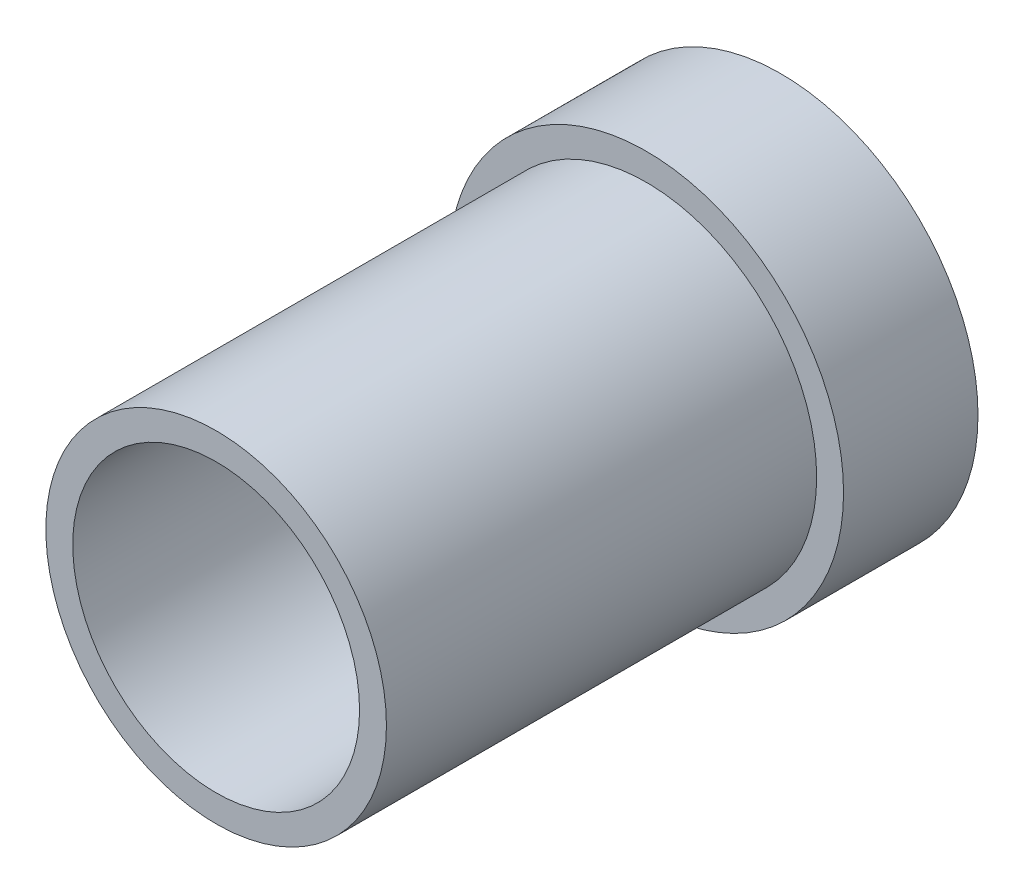
SolidWorks part; units mm, degrees
ref_plane "前视基准面" through (0, 0, 0) normal (0, 0, 1) x (1, 0, 0)
ref_plane "上视基准面" through (0, 0, 0) normal (0, 1, 0) x (1, 0, 0)
ref_plane "右视基准面" through (0, 0, 0) normal (1, 0, 0) x (0, 0, -1)
other "Configuration Table"
sketch "草图1" plane through (0, 0, 0) normal (0, 0, 1) x (1, 0, 0)
  circle A0 centre (0, 0) radius 16
  circle A1 centre (0, 0) radius 22
extrude "凸台-拉伸1" add sketch "草图1" along normal blind 15
sketch "草图2" plane through (0, 0, 15) normal (0, 0, 1) x (1, 0, 0)
  circle A0 centre (0, 0) radius 19
  circle A1 centre (0, 0) radius 16
extrude "凸台-拉伸2" add sketch "草图2" along normal blind 48
